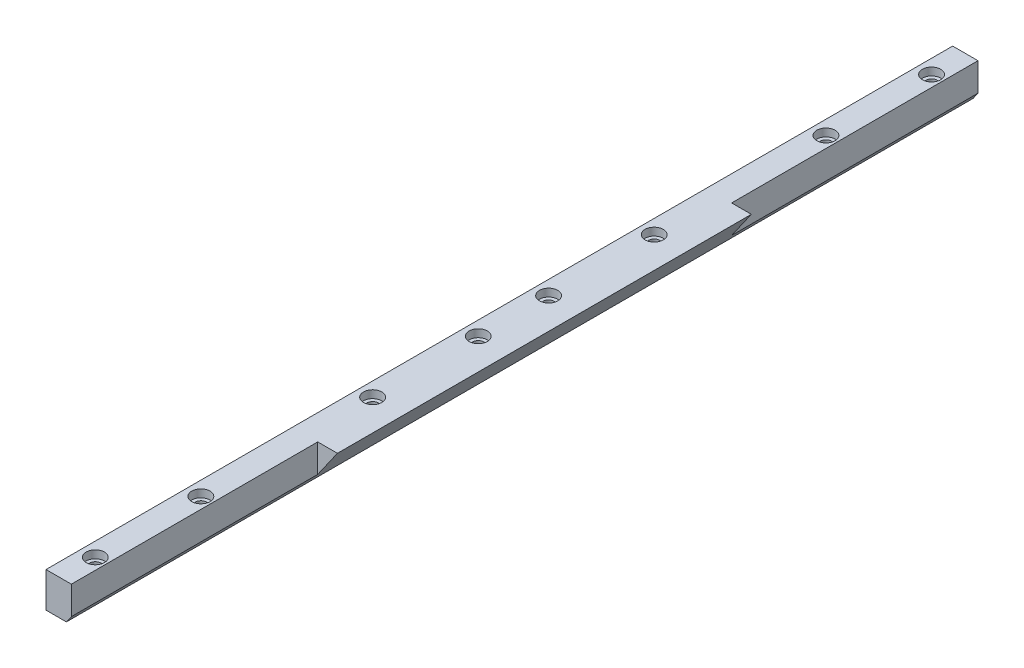
from build123d import *

# Parameters (mm, degrees)
EXTRUDE_1_DEPTH     = 1288
SKETCH_2_R          = 8
CUT_EXTRUDE_1_DEPTH = 725
SKETCH_3_R          = 13
CUT_EXTRUDE_2_DEPTH = 11
CUT_EXTRUDE_3_DEPTH = 350


with BuildPart() as part:
    # 草图1 → 凸台-拉伸1 (new body)
    with BuildSketch(Plane.XY):
        Polygon((0, 0), (0, 50), (64, 50), (29, 0), align=None)
    extrude(amount=EXTRUDE_1_DEPTH)

    # 草图2 → 切除-拉伸1 (cut)
    with BuildSketch(Plane(origin=(0, 50, 0), x_dir=(1, 0, 0), z_dir=(0, 1, 0))):
        with Locations(Location((20, -50, 0), (0, 0, 270))):
            Circle(SKETCH_2_R)
        with Locations(Location((20, -200, 0), (0, 0, 270))):
            Circle(SKETCH_2_R)
        with Locations(Location((20, -444, 0), (0, 0, 270))):
            Circle(SKETCH_2_R)
        with Locations(Location((20, -594, 0), (0, 0, 270))):
            Circle(SKETCH_2_R)
        with Locations(Location((20, -694, 0), (0, 0, 270))):
            Circle(SKETCH_2_R)
        with Locations(Location((20, -844, 0), (0, 0, 270))):
            Circle(SKETCH_2_R)
        with Locations(Location((20, -1088, 0), (0, 0, 270))):
            Circle(SKETCH_2_R)
        with Locations(Location((20, -1238, 0), (0, 0, 270))):
            Circle(SKETCH_2_R)
    extrude(amount=-CUT_EXTRUDE_1_DEPTH, mode=Mode.SUBTRACT)

    # 草图3 → 切除-拉伸2 (cut)
    with BuildSketch(Plane(origin=(0, 50, 0), x_dir=(1, 0, 0), z_dir=(0, 1, 0))):
        with Locations(Location((20, -50, 0), (0, 0, 270))):
            Circle(SKETCH_3_R)
        with Locations(Location((20, -200, 0), (0, 0, 270))):
            Circle(SKETCH_3_R)
        with Locations(Location((20, -444, 0), (0, 0, 270))):
            Circle(SKETCH_3_R)
        with Locations(Location((20, -594, 0), (0, 0, 270))):
            Circle(SKETCH_3_R)
        with Locations(Location((20, -694, 0), (0, 0, 270))):
            Circle(SKETCH_3_R)
        with Locations(Location((20, -844, 0), (0, 0, 270))):
            Circle(SKETCH_3_R)
        with Locations(Location((20, -1088, 0), (0, 0, 270))):
            Circle(SKETCH_3_R)
        with Locations(Location((20, -1238, 0), (0, 0, 270))):
            Circle(SKETCH_3_R)
    extrude(amount=-CUT_EXTRUDE_2_DEPTH, mode=Mode.SUBTRACT)

    # 草图4 → 切除-拉伸3 (cut)
    with BuildSketch(Plane.XY.offset(1288)):
        Polygon((64, 50), (36, 50), (36, 10), align=None)
    cut_extrude_3 = extrude(amount=-CUT_EXTRUDE_3_DEPTH, mode=Mode.SUBTRACT)

    # 镜向1: 切除-拉伸3 across plane
    add(cut_extrude_3.mirror(Plane(origin=(0, 0, 644), x_dir=(1, 0, 0), z_dir=(0, 0, -1))), mode=Mode.SUBTRACT)


solid = part.part
